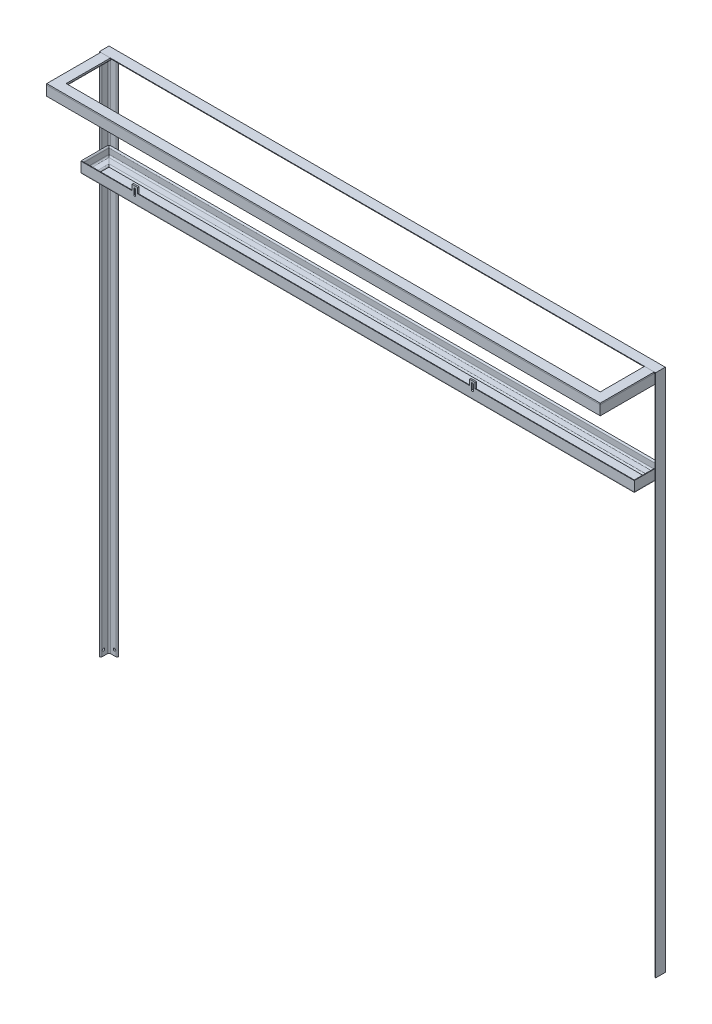
SolidWorks part; units mm, degrees
ref_plane "前视基准面" through (0, 0, 0) normal (0, 0, 1) x (1, 0, 0)
ref_plane "上视基准面" through (0, 0, 0) normal (0, 1, 0) x (1, 0, 0)
ref_plane "右视基准面" through (0, 0, 0) normal (1, 0, 0) x (0, 0, -1)
sketch "草图1" plane through (0, 0, 0) normal (0, 0, 1) x (1, 0, 0)
  line L0 (0, 0) -> (2010, 0)
  line L1 (0, 0) -> (0, -1894)
  line L2 (2010, 0) -> (2010, -1894)
  dimension "D1" = 2010
  dimension "D2" = 1894
  dimension "D3" = 1894
other "结构构件1"
ref_plane "基准面1" through (0, 0, 0) normal (1, 0, 0) x (0, 0, 1)
sketch "Sketch1" plane through (0, 0, 0) normal (1, 0, 0) x (0, 0, 1)
  line L0 (0, 0) -> (0, 35)
  line L1 (0, 17.5) -> (5, 17.5) construction
  line L2 (5, 30) -> (5, 10)
  line L3 (10, 5) -> (30, 5)
  line L4 (17.5, 5) -> (17.5, 0) construction
  line L5 (35, 0) -> (0, 0)
  arc A0 (35, 0) -> (30, 5) centre (30, 0) ccw
  arc A1 (0, 35) -> (5, 30) centre (0, 30) cw
  arc A2 (10, 5) -> (5, 10) centre (10, 10) cw
  point P10 (17.5, 0)
  point P14 (0, 17.5)
  point P15 (5, 17.5)
  point P16 (17.5, 5)
  point P17 (5, 35)
  point P18 (35, 5)
  point P21 (0, 0)
  dimension "D2" = 5
  dimension "D3" = 35
  dimension "Radius_1" = 5
  dimension "D1" = 5
sketch "草图3" plane through (0, -5, 0) normal (0, -1, 0) x (1, 0, 0)
  line L0 (5, 5) -> (5, 230)
  line L1 (2005, 5) -> (2005, 230)
  line L2 (2005, 230) -> (5, 230)
  line L3 (2005, 30) -> (2005, 10) construction
  line L4 (2000, 5) -> (1980, 5) construction
  line L5 (5, 10) -> (5, 30) construction
  dimension "D2" = 225
  dimension "D3" = 225
other "结构构件2"
ref_plane "基准面2" through (5, -5, 5) normal (0, 0, 1) x (0, -1, 0)
sketch "Sketch11" plane through (5, -5, 5) normal (0, 0, 1) x (0, -1, 0)
  line L0 (0, 0) -> (0, 35)
  line L1 (0, 17.5) -> (5, 17.5) construction
  line L2 (5, 30) -> (5, 10)
  line L3 (10, 5) -> (30, 5)
  line L4 (17.5, 5) -> (17.5, 0) construction
  line L5 (35, 0) -> (0, 0)
  arc A0 (35, 0) -> (30, 5) centre (30, 0) ccw
  arc A1 (0, 35) -> (5, 30) centre (0, 30) cw
  arc A2 (10, 5) -> (5, 10) centre (10, 10) cw
  point P10 (17.5, 0)
  point P14 (0, 17.5)
  point P15 (5, 17.5)
  point P16 (17.5, 5)
  point P17 (5, 35)
  point P18 (35, 5)
  point P21 (0, 0)
  dimension "D2" = 5
  dimension "D3" = 35
  dimension "Radius_1" = 5
  dimension "D1" = 5
ref_plane "基准面3" through (0, -339, 0) normal (0, 1, 0) x (-1, 0, 0)
sketch "草图5" plane through (0, -339, 0) normal (0, 1, 0) x (-1, 0, 0)
  line L0 (-2005, 5) -> (-2005, 107)
  line L1 (-2005, 5) -> (-2005, 230) construction
  line L2 (-2005, 107) -> (-5, 107)
  line L3 (-5, 230) -> (-5, 5) construction
  line L4 (-5, 107) -> (-5, 5)
  line L5 (-2005, 5) -> (-5, 5)
  dimension "D1" = 102
other "结构构件3"
ref_plane "基准面4" through (2005, -339, 5) normal (0, 0, 1) x (0, 1, 0)
sketch "Sketch12" plane through (2005, -339, 5) normal (0, 0, 1) x (0, 1, 0)
  line L0 (0, 0) -> (0, 35)
  line L1 (0, 17.5) -> (5, 17.5) construction
  line L2 (5, 30) -> (5, 10)
  line L3 (10, 5) -> (30, 5)
  line L4 (17.5, 5) -> (17.5, 0) construction
  line L5 (35, 0) -> (0, 0)
  arc A0 (35, 0) -> (30, 5) centre (30, 0) ccw
  arc A1 (0, 35) -> (5, 30) centre (0, 30) cw
  arc A2 (10, 5) -> (5, 10) centre (10, 10) cw
  point P10 (17.5, 0)
  point P14 (0, 17.5)
  point P15 (5, 17.5)
  point P16 (17.5, 5)
  point P17 (5, 35)
  point P18 (35, 5)
  point P21 (0, 0)
  dimension "D2" = 5
  dimension "D3" = 35
  dimension "Radius_1" = 5
  dimension "D1" = 5
sketch "草图8" plane through (0, 0, 5) normal (0, 0, 1) x (1, 0, 0)
  line L0 (35, -35) -> (35, -1894) construction
  line L1 (10, -1894) -> (30, -1894) construction
  line L2 (1005, -339) -> (1005, -2038.6334) construction
  line L3 (5, -339) -> (2005, -339) construction
  circle A0 centre (25, -1874) radius 4.5
  circle A1 centre (1985, -1874) radius 4.5
  dimension "D1" = 9
  dimension "D2" = 10
  dimension "D3" = 20
extrude "切除-拉伸1" cut sketch "草图8" against normal blind 10
sketch "草图9" plane through (0, 0, 0) normal (-1, 0, 0) x (0, 0, 1)
  line L0 (35, 0) -> (35, -1894) construction
  line L1 (0, -1894) -> (35, -1894) construction
  circle A0 centre (25, -1874) radius 4.5
  dimension "D1" = 9
  dimension "D2" = 10
  dimension "D3" = 20
extrude "切除-拉伸2" cut sketch "草图9" against normal blind 697
sketch "草图10" plane through (0, -5, 0) normal (0, 1, 0) x (1, 0, 0)
  line L0 (5, -35) -> (5, -230)
  line L1 (2010, -35) -> (0, -35) construction
  line L2 (5, -230) -> (5, -5) construction
  line L3 (40, -195) -> (5, -230) construction
  line L4 (2005, -230) -> (5, -230) construction
  line L5 (5, -230) -> (2005, -230)
  line L6 (2005, -230) -> (2005, -35)
  line L7 (2005, -35) -> (1970, -35)
  line L8 (1970, -5) -> (1970, -195) construction
  line L9 (1970, -35) -> (1970, -195)
  line L10 (1970, -195) -> (40, -195)
  line L11 (1970, -195) -> (40, -195) construction
  line L12 (40, -195) -> (40, -35)
  line L13 (40, -195) -> (40, -5) construction
  line L14 (40, -35) -> (5, -35)
extrude "凸台-拉伸1" add sketch "草图10" along normal blind 5 separate body
sketch "草图11" plane through (0, -339, 0) normal (0, -1, 0) x (1, 0, 0)
  line L0 (1970, 40) -> (2005, 5) construction
  line L1 (5, 107) -> (2005, 107)
  line L2 (5, 107) -> (5, 10)
  line L3 (10, 5) -> (2000, 5)
  line L4 (2005, 107) -> (2005, 10)
  line L5 (2005, 5) -> (1970, 40) construction
  line L6 (2005, 107) -> (2005, 5) construction
  arc A0 (10, 5) -> (5, 10) centre (10, 10) cw
  arc A1 (2005, 10) -> (2000, 5) centre (2000, 10) cw
  point P13 (2005, 5)
  dimension "D1" = 5
extrude "凸台-拉伸2" add sketch "草图11" along normal blind 2 separate body
sketch "草图13" plane through (0, 0, 107) normal (0, 0, 1) x (1, 0, 0)
  line L0 (5, -304) -> (2005, -304) construction
  line L1 (190, -284) -> (210, -284)
  line L2 (190, -284) -> (190, -314)
  line L3 (190, -314) -> (210, -314)
  line L4 (210, -284) -> (210, -314)
  line L5 (200, -284) -> (200, -356.5492) construction
  line L6 (0, 0) -> (0, -1894) construction
  line L7 (1420, -284) -> (1420, -356.5492) construction
  line L8 (1410, -284) -> (1430, -284)
  line L9 (1410, -284) -> (1410, -314)
  line L10 (1410, -314) -> (1430, -314)
  line L11 (1430, -284) -> (1430, -314)
  dimension "D1" = 20
  dimension "D2" = 30
  dimension "D3" = 10
  dimension "D4" = 200
  dimension "D5" = 20
  dimension "D6" = 30
  dimension "D7" = 10
  dimension "D8" = 1220
extrude "凸台-拉伸3" add sketch "草图13" against normal blind 5
sketch "草图12" plane through (0, 0, 107) normal (0, 0, 1) x (1, 0, 0)
  line L0 (2023.0639, -294) -> (-300.4461, -294) construction
  line L1 (196.5, -294) -> (196.5, -314)
  line L2 (203.5, -294) -> (203.5, -314)
  line L3 (210, -284) -> (190, -284) construction
  line L4 (200, -284) -> (200, -322.4048) construction
  line L5 (210, -284) -> (190, -284) construction
  line L6 (1420, -284) -> (1420, -318.2547) construction
  line L7 (1430, -284) -> (1410, -284) construction
  line L8 (1416.5, -294) -> (1416.5, -314)
  line L9 (1423.5, -294) -> (1423.5, -314)
  arc A0 (1423.5, -294) -> (1416.5, -294) centre (1420, -294) ccw
  arc A1 (203.5, -294) -> (196.5, -294) centre (200, -294) ccw
  arc A2 (1416.5, -314) -> (1423.5, -314) centre (1420, -314) ccw
  arc A3 (196.5, -314) -> (203.5, -314) centre (200, -314) ccw
  point P6 (200, -284)
  dimension "D1" = 7
  dimension "D2" = 7
  dimension "D5" = 20
  dimension "D4" = 7
  dimension "D7" = 7
  dimension "D8" = 20
  dimension "D3" = 10
  dimension "D6" = 7
  dimension "D9" = 7
extrude "切除-拉伸3" cut sketch "草图12" against normal blind 10
